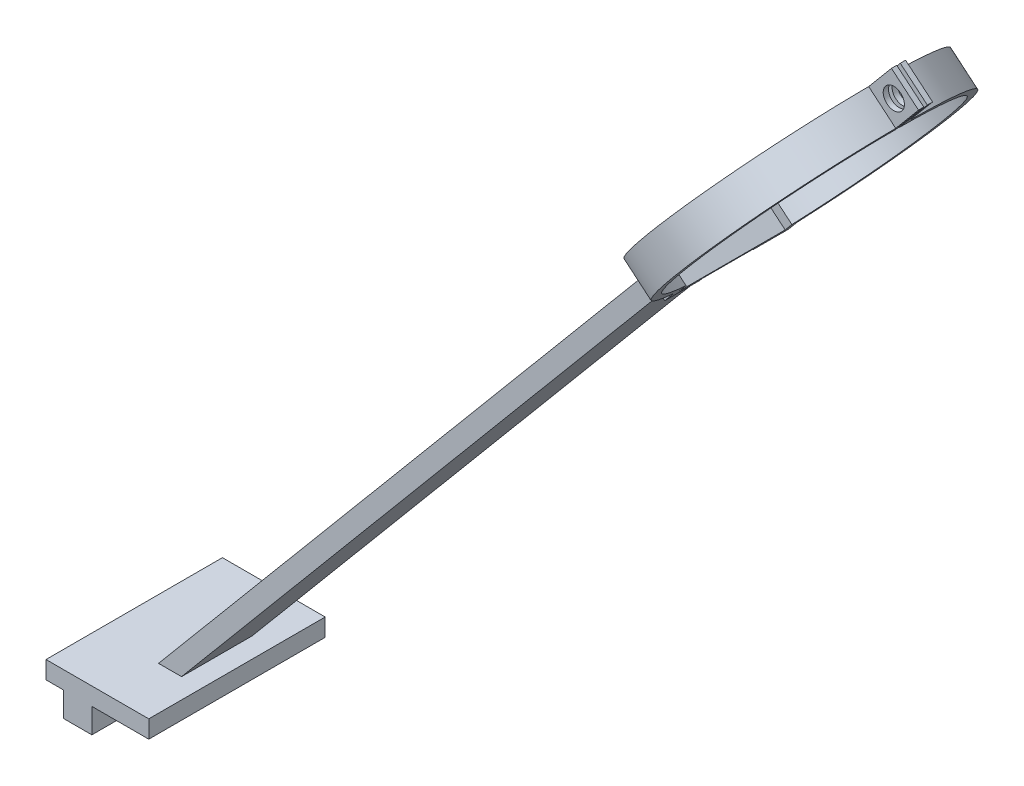
from build123d import *

# Parameters (mm, degrees)
EXTRUDE_1_DEPTH               = 10
EXTRUDE_2_DEPTH               = 5
EXTRUDE_2_DEPTH_BACK          = 5
EXTRUDE_2_START               = -2.5
CUT_EXTRUDE_3_DEPTH           = 308.667661103
CUT_EXTRUDE_3_DEPTH_BACK      = 308.667661103
SKETCH_4_W                    = 20
SKETCH_4_H                    = 2.700809371
CUT_EXTRUDE_2_DEPTH           = 308.667661103
CUT_EXTRUDE_2_DEPTH_BACK      = 308.667661103
SKETCH_5_W                    = 1
SKETCH_5_H                    = 14.903200109
SKETCH_8_W                    = 10
SKETCH_8_H                    = 1.5
EXTRUDE_2_2_DEPTH             = 10
EXTRUDE_2_2_DIRECTION_2_REACH = 314.682
SKETCH_11_W                   = 20
SKETCH_11_H                   = 26.003490823
CUT_EXTRUDE_4_DEPTH           = 10
EXTRUDE_3_DEPTH               = 15
CUT_EXTRUDE_5_DEPTH           = 318.837559332
CUT_EXTRUDE_5_DEPTH_BACK      = 318.837559332
SKETCH_13_R                   = 3
EXTRUDE_4_DEPTH               = 50


with BuildPart() as part:
    # 草图1 → 凸台-拉伸1 (new, symmetric)
    with BuildSketch(Plane.XY):
        Polygon((0, 0), (138.199336083, 164.699555271), (145.269999789, 173.126044145), (149.100222005, 169.912106096), (142.029558298, 161.485617222), (10.722534603, 5), (4.294658506, -2.660444431), (30, -2.660444431), (30, -7.660444431), (-6.427876097, -7.660444431), align=None)
    extrude(amount=EXTRUDE_1_DEPTH, both=True)

    # 草图3 → Extrude 2 (add, two sides: drawn at the far end of the back side and taken through both)
    with BuildSketch(Plane(origin=(0, 0, 0), x_dir=(0, 0, 1), z_dir=(-0.766044443118979, 0.642787609686538, 0)).offset(EXTRUDE_2_START - EXTRUDE_2_DEPTH_BACK)):
        with BuildLine():
            Line((-17.5, 226.389937847), (-17.5, 226.243201682))
            Line((-17.5, 226.243201682), (-17.5, 222.5))
            Line((-17.5, 222.5), (-7.5, 222.5))
            Line((-7.5, 222.5), (-7.5, 223.5))
            Line((-7.5, 223.5), (7.5, 223.5))
            Line((7.5, 223.5), (7.5, 222.5))
            Line((7.5, 222.5), (17.5, 222.5))
            Line((17.5, 222.5), (17.5, 226.243201682))
            Line((17.5, 226.243201682), (17.5, 226.389937847))
            ThreePointArc((17.5, 226.389937847), (0, 300.243201682), (-17.5, 226.389937847))
        make_face()
        with BuildLine():
            Line((-15, 227.967835418), (-15, 226.243201682))
            Line((-15, 226.243201682), (-15, 225))
            Line((-15, 225), (-10, 225))
            Line((-10, 225), (-10, 226))
            Line((-10, 226), (10, 226))
            Line((10, 226), (10, 225))
            Line((10, 225), (15, 225))
            Line((15, 225), (15, 226.243201682))
            Line((15, 226.243201682), (15, 227.967835418))
            ThreePointArc((15, 227.967835418), (0, 297.743201682), (-15, 227.967835418))
        make_face(mode=Mode.SUBTRACT)
    extrude(amount=EXTRUDE_2_DEPTH + EXTRUDE_2_DEPTH_BACK)

    # 草图4 → 切除-拉伸3 (cut, two sides: drawn at the far end of the back side and taken through both)
    with BuildSketch(Plane(origin=(0, 0, 0), x_dir=(0, 0, 1), z_dir=(-0.7660444431189785, 0.6427876096865388, 0)).offset(-CUT_EXTRUDE_3_DEPTH_BACK)):
        with Locations((0, 226.350404685)):
            Rectangle(SKETCH_4_W, SKETCH_4_H)
    extrude(amount=CUT_EXTRUDE_3_DEPTH + CUT_EXTRUDE_3_DEPTH_BACK, mode=Mode.SUBTRACT)

    # 草图5 → 切除-拉伸2 (cut, two sides: drawn at the far end of the back side and taken through both)
    with BuildSketch(Plane(origin=(0, 0, 0), x_dir=(0, 0, 1), z_dir=(-0.7660444431189785, 0.6427876096865388, 0)).offset(-CUT_EXTRUDE_2_DEPTH_BACK)):
        with Locations((0, 297.743201683)):
            Rectangle(SKETCH_5_W, SKETCH_5_H)
    extrude(amount=CUT_EXTRUDE_2_DEPTH + CUT_EXTRUDE_2_DEPTH_BACK, mode=Mode.SUBTRACT)

    # 草图8 → Extrude 2 2 (add)
    with BuildSketch(Plane(origin=(192.990549633, 229.997180861, 0), x_dir=(0.766044443118979, -0.6427876096865381, 0), z_dir=(0.6427876096865381, 0.766044443118979, 0))):
        with Locations((2.5, -1.25)):
            Rectangle(SKETCH_8_W, SKETCH_8_H)
    extrude_2_2 = extrude(amount=EXTRUDE_2_2_DEPTH)

    # 草图8 → Extrude 2 2 direction 2 (add, up to next)
    with BuildSketch(Plane(origin=(192.990549633, 229.997180861, 0), x_dir=(0.766044443118979, -0.6427876096865381, 0), z_dir=(0.6427876096865381, 0.766044443118979, 0)), mode=Mode.PRIVATE) as extrude_2_2_direction_2_sk1:
        with Locations((2.5, -1.25)):
            Rectangle(SKETCH_8_W, SKETCH_8_H)
    extrude_2_2_direction_2_tool1 = extrude(extrude_2_2_direction_2_sk1.sketch, amount=-EXTRUDE_2_2_DIRECTION_2_REACH, mode=Mode.PRIVATE) - part.part
    extrude_2_2_direction_2 = extrude_2_2_direction_2_tool1.solids().sort_by_distance((194.905661, 228.390212, 1.25))[0]
    add(extrude_2_2_direction_2)

    # 镜向1: Extrude 2 2, Extrude 2 2 direction 2 across plane
    add(extrude_2_2.mirror(Plane.XY))
    add(extrude_2_2_direction_2.mirror(Plane.XY))

    # 草图11 → 切除-拉伸4 (cut)
    with BuildSketch(Plane.XZ.offset(7.660444431)):
        with Locations((20, -3.001745411)):
            Rectangle(SKETCH_11_W, SKETCH_11_H)
    extrude(amount=-CUT_EXTRUDE_4_DEPTH, mode=Mode.SUBTRACT)

    # 草图12 → 凸台-拉伸3 (add)
    with BuildSketch(Plane.XY.offset(10)):
        Polygon((4.294658506, -2.660444431), (-2.232377941, -2.660444431), (-6.427876097, -7.660444431), (10, -7.660444431), (10, -2.660444431), align=None)
    extrude_3 = extrude(amount=EXTRUDE_3_DEPTH)

    # 镜向2: 凸台-拉伸3 across plane
    add(extrude_3.mirror(Plane.XY))

    # 草图13 → 切除-拉伸5 (cut, two sides: drawn at the far end of the back side and taken through both)
    with BuildSketch(Plane(origin=(0, 0, -2), x_dir=(-1, 0, 0), z_dir=(0, 0, -1)).offset(-CUT_EXTRUDE_5_DEPTH_BACK)):
        with Locations((-198.163787282, 232.207589437)):
            Circle(SKETCH_13_R)
    extrude(amount=CUT_EXTRUDE_5_DEPTH + CUT_EXTRUDE_5_DEPTH_BACK, mode=Mode.SUBTRACT)

    # 草图14 → 凸台-拉伸4 (add)
    with BuildSketch(Plane(origin=(0, 0, -25), x_dir=(-1, 0, 0), z_dir=(0, 0, -1))):
        Polygon((2.232377941, -2.660444431), (6.427876097, -2.660444431), (14.127876097, -2.660444431), (19.127876097, -2.660444431), (19.127876097, -7.660444431), (14.127876097, -7.660444431), (14.127876097, -14.660444431), (6.427876097, -14.660444431), (6.127876097, -14.660444431), (6.127876097, -7.660444431), (6.427876097, -7.660444431), align=None)
    extrude(amount=-EXTRUDE_4_DEPTH)


solid = part.part
